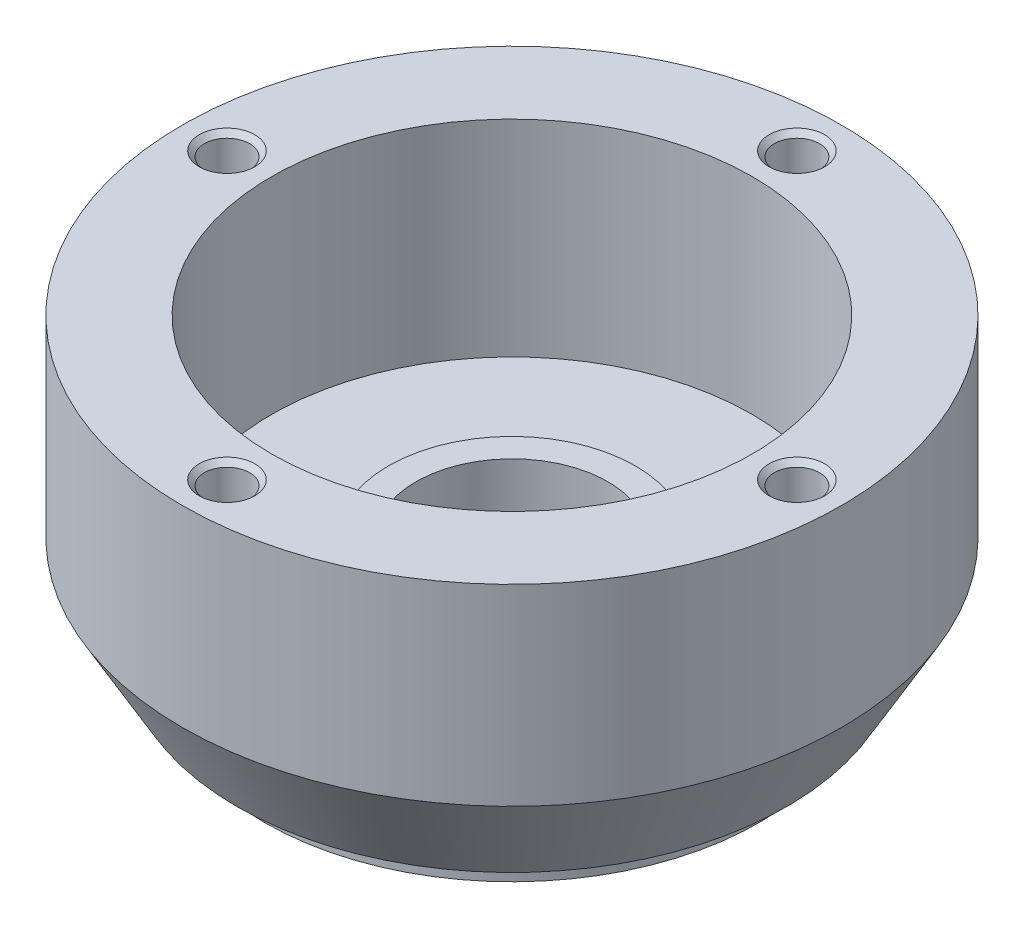
from build123d import *

# Parameters (mm, degrees)
SKETCH2_R           = 17.5
CUT_EXTRUDE1_DEPTH  = 15
SKETCH3_R           = 9
BOSS_EXTRUDE1_DEPTH = 1
SKETCH4_R           = 7
CUT_EXTRUDE2_DEPTH  = 37.715119501
SKETCH5_R           = 2
CUT_EXTRUDE3_DEPTH  = 4
CIRPATTERN1_COUNT   = 8
CIRPATTERN2_COUNT   = 4
CHAMFER1_SIZE       = 0.5


with BuildPart() as part:
    # Sketch1 → Revolve1 (revolve)
    with BuildSketch(Plane(origin=(0, 0, 0), x_dir=(0, 0, -1), z_dir=(1, 0, 0))):
        Polygon((0, 0), (-18, 0), (-18, 2), (-20, 2), (-24, 9), (-24, 23), (0, 23), align=None)
    revolve(axis=Axis((0, 23, 0), (0, -1, 0)))

    # Sketch2 → Cut-Extrude1 (cut)
    with BuildSketch(Plane(origin=(0, 23, 0), x_dir=(1, 0, 0), z_dir=(0, 1, 0))):
        with Locations(Location((0, 0, 0), (0, 0, 270))):
            Circle(SKETCH2_R)
    extrude(amount=-CUT_EXTRUDE1_DEPTH, mode=Mode.SUBTRACT)

    # Sketch3 → Boss-Extrude1 (add)
    with BuildSketch(Plane(origin=(0, 8, 0), x_dir=(1, 0, 0), z_dir=(0, 1, 0))):
        with Locations(Location((0, 0, 0), (0, 0, 270))):
            Circle(SKETCH3_R)
    extrude(amount=BOSS_EXTRUDE1_DEPTH)

    # Sketch4 → Cut-Extrude2 (cut, through all)
    with BuildSketch(Plane(origin=(0, 9, 0), x_dir=(1, 0, 0), z_dir=(0, 1, 0))):
        with Locations(Location((0, 0, 0), (0, 0, 270))):
            Circle(SKETCH4_R)
    extrude(amount=-CUT_EXTRUDE2_DEPTH, mode=Mode.SUBTRACT)

    # Sketch5 → Cut-Extrude3 (cut)
    with BuildSketch(Plane.XZ):
        with Locations(Location((0, 14, 0), (0, 0, 270))):
            Circle(SKETCH5_R)
    extrude(amount=-CUT_EXTRUDE3_DEPTH, mode=Mode.SUBTRACT)

    # Sketch6 → Cut-Revolve1 (revolve, cut)
    with BuildSketch(Plane.XY):
        with BuildLine():
            Line((-16, 0), (-14, 0))
            Line((-14, 0), (-14, 1))
            ThreePointArc((-14, 1), (-15.104156256, 0.708312513), (-16, 0))
        make_face()
    cut_revolve1 = revolve(axis=Axis((-14, 0, 0), (0, 1, 0)), mode=Mode.SUBTRACT)

    # CirPattern1: Cut-Revolve1 ×8 about axis, 2 skipped
    cirpattern1_axis = Axis((0, 0, 0), (0, 1, 0))
    add([cut_revolve1.rotate(cirpattern1_axis, i * 360 / CIRPATTERN1_COUNT) for i in range(1, CIRPATTERN1_COUNT) if i not in (2, 6)], mode=Mode.SUBTRACT)

    # Sketch8 → M4 Tapped Hole1 (revolve, cut)
    with BuildSketch(Plane(origin=(0, 23, -20.75), x_dir=(0, 0, 1), z_dir=(1, 0, 0))):
        Polygon((0, 0), (0, 8.991420021), (1.65, 8), (1.65, 0.375), (2.025, 0), align=None)
    m4_tapped_hole1 = revolve(axis=Axis((0, 29.35, -20.75), (0, -1, 0)), mode=Mode.SUBTRACT)

    # CirPattern2: M4 Tapped Hole1 ×4 about axis
    cirpattern2_axis = Axis((0, 0, 0), (0, 1, 0))
    for i in range(1, CIRPATTERN2_COUNT):
        add(m4_tapped_hole1.rotate(cirpattern2_axis, i * 360 / CIRPATTERN2_COUNT), mode=Mode.SUBTRACT)

    # Chamfer1
    chamfer1_edges = [part.edges().sort_by_distance(p)[0] for p in [
        (0, 0, -7),
    ]]
    chamfer(chamfer1_edges, length=CHAMFER1_SIZE)


solid = part.part
